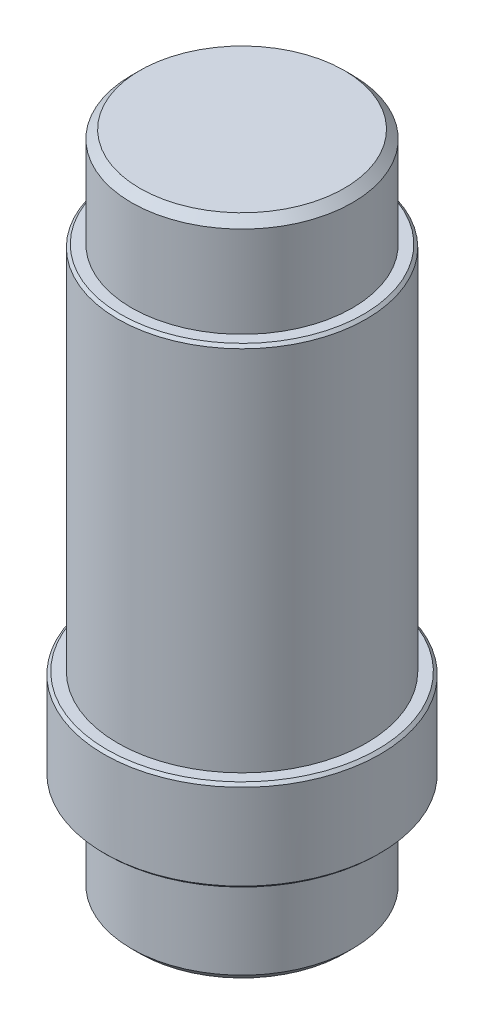
SolidWorks part; units mm, degrees
ref_plane "Front Plane" through (0, 0, 0) normal (0, 0, 1) x (1, 0, 0)
ref_plane "Top Plane" through (0, 0, 0) normal (0, 1, 0) x (1, 0, 0)
ref_plane "Right Plane" through (0, 0, 0) normal (1, 0, 0) x (0, 0, -1)
other "Configuration Table"
sketch "Sketch1" plane through (0, 0, 0) normal (0, 1, 0) x (1, 0, 0)
  circle A0 centre (0, 0) radius 50
  dimension "D1" = 100
extrude "Boss-Extrude1" add sketch "Sketch1" along normal mid plane 240
sketch "Sketch2" plane through (0, 120, 0) normal (0, 1, 0) x (1, 0, 0)
  circle A0 centre (0, 0) radius 40
  circle A1 centre (0, 0) radius 50
  dimension "D1" = 80
  dimension "D2" = 100
extrude "Cut-Extrude1" cut sketch "Sketch2" against normal blind 36
sketch "Sketch3" plane through (0, -120, 0) normal (0, -1, 0) x (1, 0, 0)
  circle A0 centre (0, 0) radius 40
  circle A1 centre (0, 0) radius 50
  dimension "D1" = 80
  dimension "D2" = 100
extrude "Cut-Extrude2" cut sketch "Sketch3" against normal blind 37
sketch "Sketch4" plane through (0, 84, 0) normal (0, 1, 0) x (1, 0, 0)
  circle A0 centre (0, 0) radius 45
  circle A1 centre (0, 0) radius 50
  dimension "D1" = 90
  dimension "D2" = 100
extrude "Cut-Extrude3" cut sketch "Sketch4" against normal blind 134
chamfer "Chamfer1" distance 3 angle 45 2 edges at (0, -120, -40) (0, 120, 40)
chamfer "Chamfer2" distance 1 angle 45 3 edges at (0, -50, 50) (0, -83, -50) (0, 84, 45)
